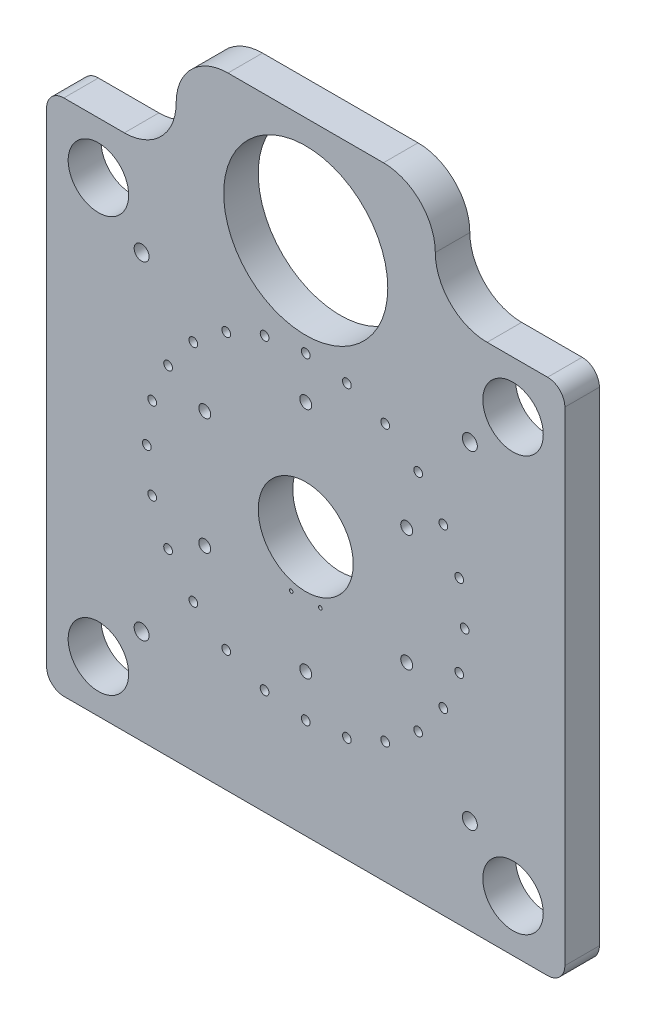
SolidWorks part; units mm, degrees
ref_plane "Front Plane" through (0, 0, 0) normal (0, 0, 1) x (1, 0, 0)
ref_plane "Top Plane" through (0, 0, 0) normal (0, 1, 0) x (1, 0, 0)
ref_plane "Right Plane" through (0, 0, 0) normal (1, 0, 0) x (0, 0, -1)
sketch "Sketch1" plane through (0, 0, 0) normal (0, 0, 1) x (1, 0, 0)
  line L0 (-96.2506, 420) -> (83.7494, 420)
  line L1 (-286.2506, 300) -> (-216.2506, 300)
  line L2 (-306.2506, -280) -> (-306.2506, 280)
  line L3 (273.7494, -300) -> (-286.2506, -300)
  line L4 (293.7494, 280) -> (293.7494, -280)
  line L5 (203.7494, 300) -> (273.7494, 300)
  circle A0 centre (-246.2506, 240) radius 49
  circle A1 centre (233.7494, -240) radius 49
  circle A2 centre (-246.2506, -240) radius 49
  circle A3 centre (233.7494, 240) radius 49
  circle A4 centre (-6.2506, 0) radius 55
  circle A5 centre (-6.2506, -184) radius 5.053
  circle A6 centre (-53.8734, -177.7304) radius 5.053
  circle A7 centre (-98.2506, -159.3487) radius 5.053
  circle A8 centre (-136.3583, -130.1076) radius 5.053
  circle A9 centre (-165.5993, -92) radius 5.053
  circle A10 centre (-183.981, -47.6227) radius 5.053
  circle A11 centre (-190.2506, 0) radius 5.053
  circle A12 centre (-183.981, 47.6227) radius 5.053
  circle A13 centre (-165.5993, 92) radius 5.053
  circle A14 centre (-136.3583, 130.1076) radius 5.053
  circle A15 centre (-98.2506, 159.3487) radius 5.053
  circle A16 centre (-53.8734, 177.7304) radius 5.053
  circle A17 centre (-6.2506, 184) radius 5.053
  circle A18 centre (41.3721, 177.7304) radius 5.053
  circle A19 centre (85.7494, 159.3487) radius 5.053
  circle A20 centre (123.857, 130.1076) radius 5.053
  circle A21 centre (153.098, 92) radius 5.053
  circle A22 centre (171.4797, 47.6227) radius 5.053
  circle A23 centre (177.7494, 0) radius 5.053
  circle A24 centre (171.4797, -47.6227) radius 5.053
  circle A25 centre (153.098, -92) radius 5.053
  circle A26 centre (123.857, -130.1076) radius 5.053
  circle A27 centre (85.7494, -159.3487) radius 5.053
  circle A28 centre (41.3721, -177.7304) radius 5.053
  circle A29 centre (-6.2506, 297) radius 95
  circle A30 centre (-6.2506, 135) radius 6.9175
  circle A31 centre (110.6628, 67.5) radius 6.9175
  circle A32 centre (110.6628, -67.5) radius 6.9175
  circle A33 centre (-6.2506, -135) radius 6.9175
  circle A34 centre (-123.1641, -67.5) radius 6.9175
  circle A35 centre (-123.1641, 67.5) radius 6.9175
  circle A36 centre (-196.2506, 190) radius 8.647
  circle A37 centre (183.7494, -190) radius 8.647
  circle A38 centre (-196.2506, -190) radius 8.647
  circle A39 centre (183.7494, 190) radius 8.647
  circle A40 centre (-23.0739, -62.7852) radius 2.067
  circle A41 centre (10.5726, -62.7852) radius 2.067
  arc A42 (-96.2506, 420) -> (-156.2506, 360) centre (-96.2506, 360) ccw
  arc A43 (-216.2506, 300) -> (-156.2506, 360) centre (-216.2506, 360) ccw
  arc A44 (-286.2506, 300) -> (-306.2506, 280) centre (-286.2506, 280) ccw
  arc A45 (-306.2506, -280) -> (-286.2506, -300) centre (-286.2506, -280) ccw
  arc A46 (273.7494, -300) -> (293.7494, -280) centre (273.7494, -280) ccw
  arc A47 (293.7494, 280) -> (273.7494, 300) centre (273.7494, 280) ccw
  arc A48 (143.7494, 360) -> (203.7494, 300) centre (203.7494, 360) ccw
  arc A49 (143.7494, 360) -> (83.7494, 420) centre (83.7494, 360) ccw
  dimension "D1" = 98
extrude "Boss-Extrude1" add sketch "Sketch1" along normal blind 40
sketch "Sketch2" plane through (0, 0, 40) normal (0, 0, 1) x (1, 0, 0)
  circle A0 centre (-246.2506, 240) radius 49
  circle A1 centre (-246.2506, 240) radius 35
  circle A2 centre (233.7494, 240) radius 49
  circle A3 centre (233.7494, 240) radius 35
  circle A4 centre (233.7494, -240) radius 49
  circle A5 centre (233.7494, -240) radius 35
  circle A6 centre (-246.2506, -240) radius 49
  circle A7 centre (-246.2506, -240) radius 35
  dimension "D1" = 98
  dimension "D2" = 70
extrude "Boss-Extrude2" add sketch "Sketch2" against normal blind 38
sketch "Sketch3" plane through (0, 0, 2) normal (0, 0, -1) x (-1, 0, 0)
  circle A0 centre (-233.7494, 240) radius 41 construction
  circle A1 centre (-192.7494, 240) radius 7.2884
  circle A2 centre (-254.2494, 204.493) radius 7.2884
  circle A3 centre (-254.2494, 275.507) radius 7.2884
  point P11 (-233.7494, 240)
  dimension "D1" = 82
  dimension "D2" = 3
hole_wizard "Size mm Dowel hole 1" positions "Sketch4" profile "Sketch5" hole size "Ø3.0" standard "GB"
sketch "Sketch4" plane through (0, 0, 2) normal (0, 0, -1) x (-1, 0, 0)
  point P0 (-254.2494, 275.507)
  point P3 (-192.7494, 240)
  point P6 (-254.2494, 204.493)
sketch "Sketch5" plane through (254.2494, 275.507, 2) normal (1, 0, 0) x (0, 1, 0)
  line L0 (0, 0) -> (0, 12.7614)
  line L1 (0, 12.7614) -> (1.6, 11.8)
  line L2 (1.6, 11.8) -> (1.6, 0)
  line L5 (1.6, 0) -> (0, 0)
  line L10 (0, 12.7614) -> (-1.6, 11.8) construction
  line L11 (0, -6.35) -> (0, 107.95) construction
  dimension "孔直径" = 3.2
  dimension "孔深度" = 11.8
  dimension "导头角度" = 118
ref_plane "Plane2" through (-6.2506, 0, 0) normal (1, 0, 0) x (0, 0, -1)
pattern_linear "LPattern1" count 2 spacing 480 along (-1, 0, 0) count 2 spacing 480 along (0, -1, 0) of "Size mm Dowel hole 1"
